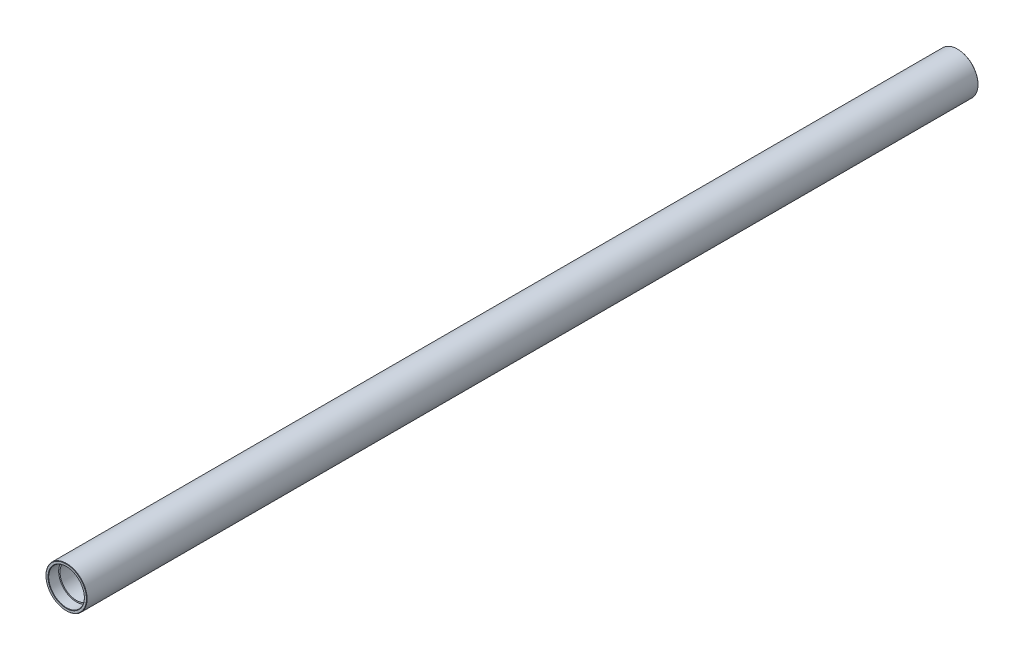
from build123d import *

# Parameters (mm, degrees)
SKETCH_1_R          = 30
EXTRUDE_1_DEPTH     = 1300
SKETCH_2_R          = 24
CUT_EXTRUDE_1_DEPTH = 1600
SKETCH_3_R          = 26
CUT_EXTRUDE_2_DEPTH = 15
CUT_EXTRUDE_START   = -15
SKETCH_4_R          = 26
CUT_EXTRUDE_3_DEPTH = 15
CHAMFER_1_SIZE      = 0.5


with BuildPart() as part:
    # 草图1 → 凸台-拉伸1 (new body)
    with BuildSketch(Plane.XY):
        Circle(SKETCH_1_R)
    extrude(amount=EXTRUDE_1_DEPTH)

    # 草图2 → 切除-拉伸1 (cut)
    with BuildSketch(Plane(origin=(0, 0, 0), x_dir=(-1, 0, 0), z_dir=(0, 0, -1))):
        Circle(SKETCH_2_R)
    extrude(amount=-CUT_EXTRUDE_1_DEPTH, mode=Mode.SUBTRACT)

    # 草图3 → 切除-拉伸2 (cut)
    with BuildSketch(Plane(origin=(0, 0, 0), x_dir=(-1, 0, 0), z_dir=(0, 0, -1))):
        Circle(SKETCH_3_R)
    extrude(amount=-CUT_EXTRUDE_2_DEPTH, mode=Mode.SUBTRACT)

    # 草图4 → 切除-拉伸3 (cut)
    with BuildSketch(Plane.XY.offset(1300).offset(CUT_EXTRUDE_START)):
        with Locations(Location((0, 0, 0), (0, 0, 180))):
            Circle(SKETCH_4_R)
    extrude(amount=CUT_EXTRUDE_3_DEPTH, mode=Mode.SUBTRACT)

    # 倒角1
    chamfer_1_edges = [part.edges().sort_by_distance(p)[0] for p in [
        (26, 0, 0),
        (-30, 0, 0),
        (26, 0, 1300),
        (-30, 0, 1300),
    ]]
    chamfer(chamfer_1_edges, length=CHAMFER_1_SIZE)


solid = part.part
